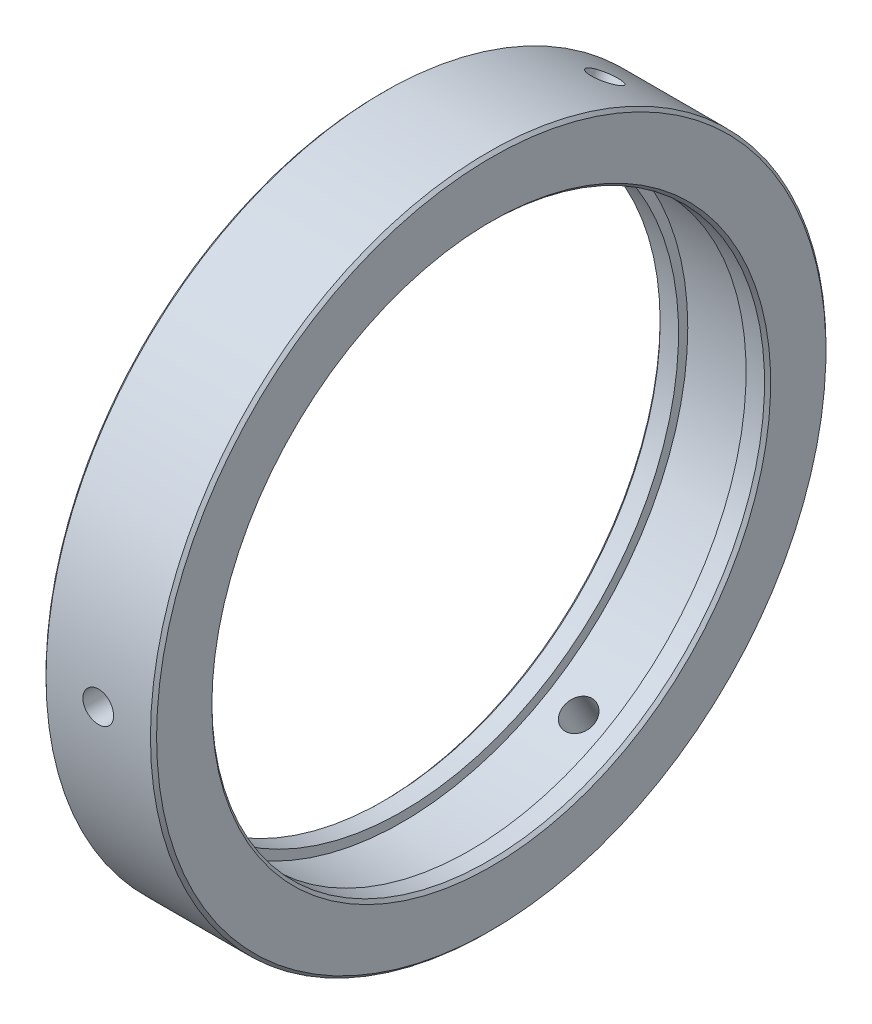
from build123d import *

# Parameters (mm, degrees)
CHAMFER1_SIZE     = 1
HOLE1_D           = 10
HOLE1_DEPTH       = 18
CIRPATTERN1_COUNT = 3


with BuildPart() as part:
    # Sketch2 → Revolve1 (revolve)
    with BuildSketch(Plane.XY, mode=Mode.PRIVATE) as revolve1_sk:
        Polygon((-18, 90), (-18, 110), (18, 110), (18, 90), (11, 90), (11, 93), (-11, 93), (-11, 90), align=None)
    revolve(revolve1_sk.sketch.rotate(Axis((-24.332542805, 0, 0), (1, 0, 0)), 90), axis=Axis((-24.332542805, 0, 0), (1, 0, 0)))

    # Chamfer1
    chamfer1_edges = [part.edges().sort_by_distance(p)[0] for p in [
        (-18, 0, -110),
        (-18, 0, -90),
        (18, 0, -90),
        (18, 0, -110),
    ]]
    chamfer(chamfer1_edges, length=CHAMFER1_SIZE)

    # Hole1
    with Locations(Plane.XY.offset(110)):
        with Locations((0, 0)):
            hole1 = Hole(HOLE1_D / 2, depth=HOLE1_DEPTH)

    # CirPattern1: Hole1 ×3 about axis
    cirpattern1_axis = Axis((17, 0, 0), (-1, 0, 0))
    for i in range(1, CIRPATTERN1_COUNT):
        add(hole1.rotate(cirpattern1_axis, i * 360 / CIRPATTERN1_COUNT), mode=Mode.SUBTRACT)


solid = part.part
